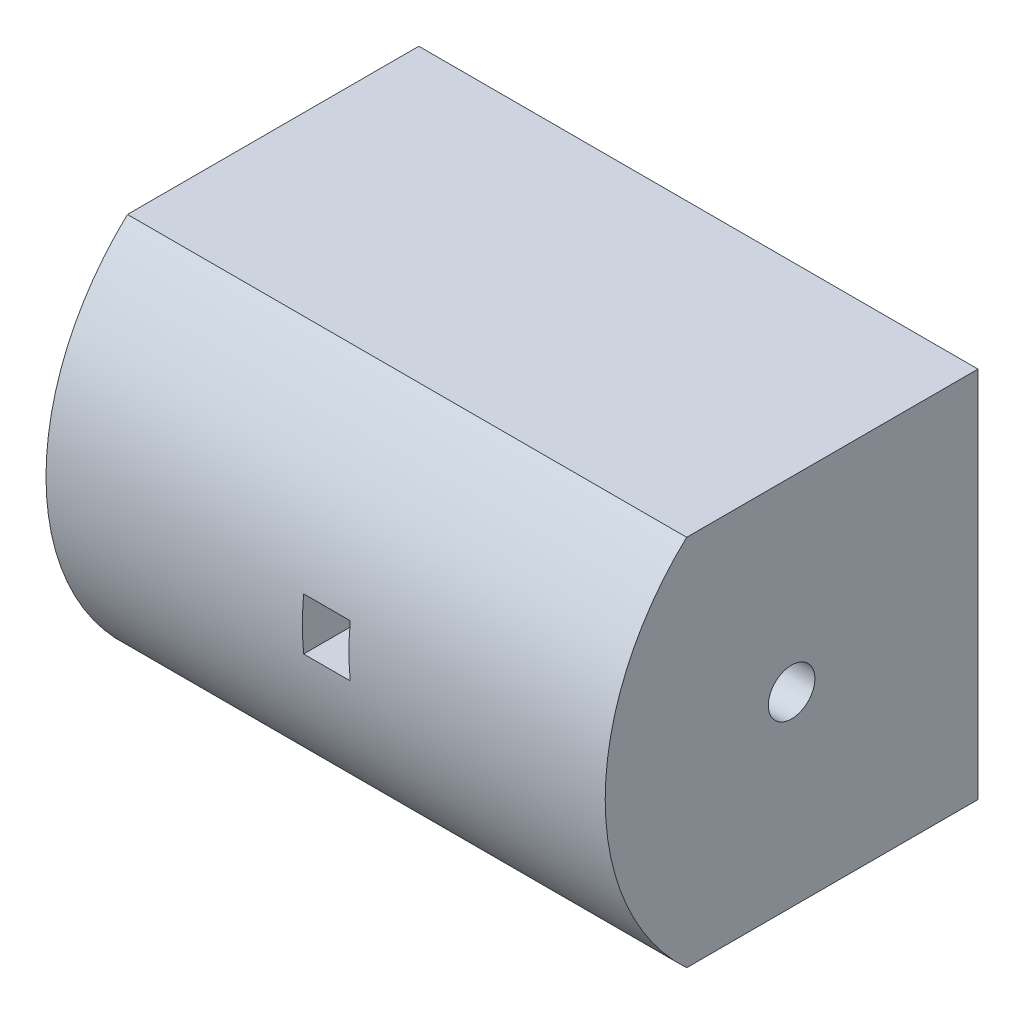
from build123d import *

# Parameters (mm, degrees)
SKETCH_1_W          = 120
SKETCH_1_H          = 80
EXTRUDE_1_DEPTH     = 80
SKETCH_2_R          = 5
CUT_EXTRUDE_1_DEPTH = 150.666295471
CUT_EXTRUDE_2_DEPTH = 150.666295471
CUT_EXTRUDE_3_REACH = 109.703
SKETCH_5_W          = 10
SKETCH_5_H          = 11.18
SKETCH_6_W          = 10
SKETCH_6_H          = 11.18
EXTRUDE_2_DEPTH     = 50


with BuildPart() as part:
    # 草图1 → 凸台-拉伸1 (new body)
    with BuildSketch(Plane.XY):
        Rectangle(SKETCH_1_W, SKETCH_1_H)
    extrude(amount=EXTRUDE_1_DEPTH)

    # 草图2 → 切除-拉伸1 (cut, through all)
    with BuildSketch(Plane.ZY.offset(60)):
        with Locations((40, 0)):
            Circle(SKETCH_2_R)
    extrude(amount=-CUT_EXTRUDE_1_DEPTH, mode=Mode.SUBTRACT)

    # 草图4 → 切除-拉伸2 (cut, through all)
    with BuildSketch(Plane(origin=(60, 0, 0), x_dir=(0, 0, -1), z_dir=(1, 0, 0))):
        with BuildLine():
            ThreePointArc((-80, 4.27e-07), (-75.438313853, 21.82692854), (-62.516888038, 40))
            Line((-62.516888038, 40), (-80, 40))
            Line((-80, 40), (-80, 4.27e-07))
        make_face()
        with BuildLine():
            ThreePointArc((-62.516888038, -40), (-75.438314024, -21.826928149), (-80, 4.27e-07))
            Line((-80, 4.27e-07), (-80, -40))
            Line((-80, -40), (-62.516888038, -40))
        make_face()
    extrude(amount=-CUT_EXTRUDE_2_DEPTH, mode=Mode.SUBTRACT)

    # 草图5 → 切除-拉伸3 (cut, up to next)
    with BuildSketch(Plane(origin=(0, 0, 0), x_dir=(-1, 0, 0), z_dir=(0, 0, -1)), mode=Mode.PRIVATE) as cut_extrude_3_sk1:
        Rectangle(SKETCH_5_W, SKETCH_5_H)
    cut_extrude_3_tool1 = extrude(cut_extrude_3_sk1.sketch, amount=-CUT_EXTRUDE_3_REACH, mode=Mode.PRIVATE) & part.part
    add(cut_extrude_3_tool1.solids().sort_by_distance((0, 0, 0))[0], mode=Mode.SUBTRACT)

    # 草图6 → 凸台-拉伸2 (add)
    with BuildSketch(Plane(origin=(0, 0, 0), x_dir=(-1, 0, 0), z_dir=(0, 0, -1))):
        Rectangle(SKETCH_6_W, SKETCH_6_H)
    extrude(amount=-EXTRUDE_2_DEPTH)


solid = part.part
